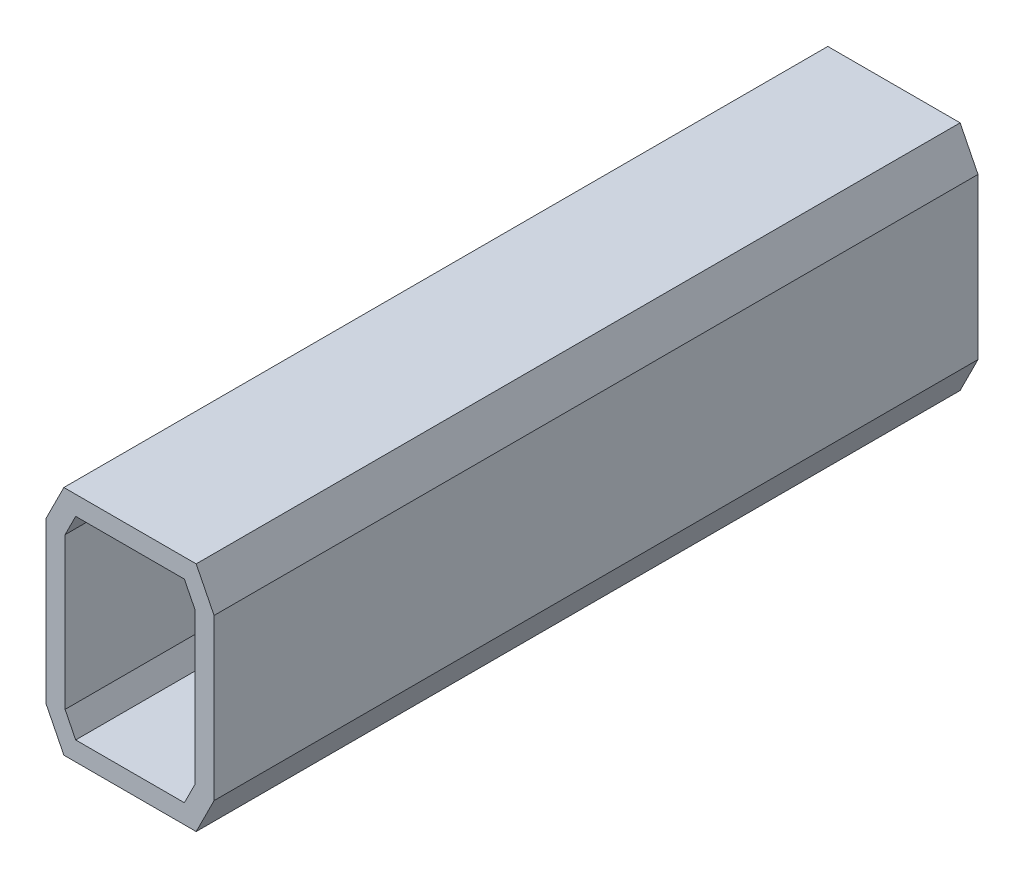
from build123d import *

# Parameters (mm, degrees)
BOSS_EXTRUDE1_DEPTH = 200


with BuildPart() as part:
    # Sketch1 → Boss-Extrude1 (new body)
    with BuildSketch(Plane.XY):
        Polygon((-17.319660113, 136.5), (17.319660113, 136.5), (22, 127.139320225), (22, 85.160679775), (17.319660113, 75.8), (-17.319660113, 75.8), (-22, 85.160679775), (-22, 127.139320225), align=None)
        Polygon((-14.229490169, 131.5), (14.229490169, 131.5), (17, 125.958980338), (17, 86.341019662), (14.229490169, 80.8), (-14.229490169, 80.8), (-17, 86.341019662), (-17, 125.958980338), align=None, mode=Mode.SUBTRACT)
    extrude(amount=BOSS_EXTRUDE1_DEPTH)


solid = part.part
